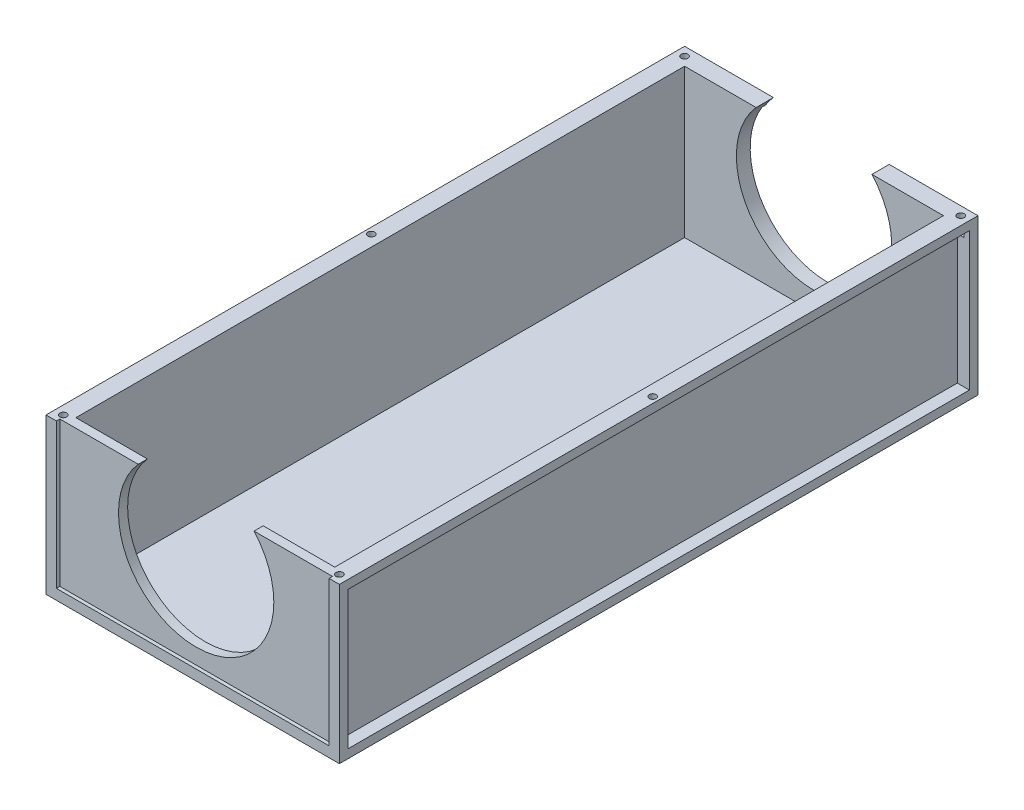
from build123d import *

# Parameters (mm, degrees)
SKETCH_1_R           = 50
SKETCH_1_R_2         = 42.55
EXTRUDE_1_DEPTH      = 50
SKETCH_3_R           = 45
SKETCH_3_R_2         = 37.55
EXTRUDE_2_DEPTH      = 50
EXTRUDE_START        = -50
EXTRUDE_3_DEPTH      = 50
SKETCH_8_R           = 37.55
EXTRUDE_4_DEPTH      = 50
SKETCH_4_W           = 700
SKETCH_4_H           = 3700
EXTRUDE_5_DEPTH      = 300
SKETCH_12_W          = 500
SKETCH_12_H          = 1000
EXTRUDE_6_DEPTH      = 300
SKETCH_16_W          = 500
SKETCH_16_H          = 2700
EXTRUDE_8_DEPTH      = 300
SKETCH_17_W          = 100
SKETCH_17_H          = 100
EXTRUDE_9_DEPTH      = 600
SKETCH_18_W          = 100
SKETCH_18_H          = 100
EXTRUDE_10_DEPTH     = 600
SKETCH_19_W          = 100
SKETCH_19_H          = 100
EXTRUDE_11_DEPTH     = 3500
SKETCH_20_R          = 25
CUT_EXTRUDE_5_DEPTH  = 20
SKETCH_21_R          = 52.5
SKETCH_21_R_2        = 42.55
EXTRUDE_12_DEPTH     = 50
CUT_EXTRUDE_START    = -356
CUT_EXTRUDE_6_DEPTH  = 356
SKETCH_23_W          = 47.45
SKETCH_23_H          = 50
EXTRUDE_13_DEPTH     = 20
CUT_EXTRUDE_8_DEPTH  = 611
SKETCH_26_W          = 52.45
SKETCH_26_H          = 50
EXTRUDE_14_DEPTH     = 20
SKETCH_27_R          = 6
CUT_EXTRUDE_9_DEPTH  = 20
SKETCH_28_R          = 6
CUT_EXTRUDE_10_DEPTH = 20
EXTRUDE_START_2      = -53
EXTRUDE_15_DEPTH     = 53
EXTRUDE_START_3      = 3
EXTRUDE_16_DEPTH     = 3
EXTRUDE_17_DEPTH     = 3
EXTRUDE_18_DEPTH     = 53
SKETCH_31_W          = 3500
SKETCH_31_H          = 500
EXTRUDE_19_DEPTH     = 100
SKETCH_33_W          = 500
SKETCH_33_H          = 3700
EXTRUDE_20_DEPTH     = 300
EXTRUDE_21_DEPTH     = 100
SKETCH_35_W          = 1500
SKETCH_35_H          = 600
EXTRUDE_22_DEPTH     = 100
SKETCH_36_W          = 1500
SKETCH_36_H          = 600
EXTRUDE_23_DEPTH     = 100
SKETCH_37_W          = 3600
SKETCH_37_H          = 800
CUT_EXTRUDE_11_DEPTH = 70
SKETCH_38_W          = 1580
SKETCH_38_H          = 780
CUT_EXTRUDE_15_DEPTH = 20
SKETCH_39_W          = 3600
SKETCH_39_H          = 800
CUT_EXTRUDE_16_DEPTH = 70
SKETCH_40_W          = 1580
SKETCH_40_H          = 780
CUT_EXTRUDE_17_DEPTH = 20
SKETCH_43_R          = 20
CUT_EXTRUDE_20_DEPTH = 100
CUT_EXTRUDE_22_DEPTH = 260
SKETCH_44_W          = 1500
SKETCH_44_H          = 3527
CUT_EXTRUDE_24_DEPTH = 983
CUT_EXTRUDE_25_DEPTH = 260
SKETCH_49_W          = 1580
SKETCH_49_H          = 840
CUT_EXTRUDE_26_DEPTH = 20
SKETCH_52_R          = 450
CUT_EXTRUDE_30_DEPTH = 492
SKETCH_53_R          = 450
CUT_EXTRUDE_31_DEPTH = 492


with BuildPart() as part:
    # 草图1 → 凸台-拉伸1 (new body)
    with BuildSketch(Plane.XY):
        Circle(SKETCH_1_R)
        Circle(SKETCH_1_R_2, mode=Mode.SUBTRACT)
    extrude(amount=EXTRUDE_1_DEPTH)

    # 草图7 → 凸台-拉伸3 (add)
    with BuildSketch(Plane.XY.offset(50).offset(EXTRUDE_START)):
        with BuildLine():
            ThreePointArc((50, 0), (0, -50), (-50, 0))
            Line((-50, 0), (-250, -900))
            Line((-250, -900), (250, -900))
            Line((250, -900), (50, 0))
        make_face()
    extrude(amount=EXTRUDE_3_DEPTH)



with BuildPart() as body_2:
    # 草图3 → 凸台-拉伸2 (new body)
    with BuildSketch(Plane(origin=(0, 0, -3374), x_dir=(-1, 0, 0), z_dir=(0, 0, -1))):
        Circle(SKETCH_3_R)
        Circle(SKETCH_3_R_2, mode=Mode.SUBTRACT)
    extrude(amount=EXTRUDE_2_DEPTH)

    # 草图8 → 凸台-拉伸4 (add)
    with BuildSketch(Plane(origin=(0, 0, -3424), x_dir=(-1, 0, 0), z_dir=(0, 0, -1))):
        with BuildLine():
            Line((-43.888190419, 9.941164005), (-250, -900))
            Line((-250, -900), (250, -900))
            Line((250, -900), (43.888190419, 9.941164005))
            ThreePointArc((43.888190419, 9.941164005), (0, 45), (-43.888190419, 9.941164005))
        make_face()
        Circle(SKETCH_8_R, mode=Mode.SUBTRACT)
    extrude(amount=-EXTRUDE_4_DEPTH)


with BuildPart() as part_1:
    add(part.part)

    add(body_2.part)  # 凸台-拉伸5 merges body 2
    # 草图4 → 凸台-拉伸5 (add)
    with BuildSketch(Plane(origin=(0, -900, 0), x_dir=(1, 0, 0), z_dir=(0, 1, 0))):
        with Locations((0, 1724)):
            Rectangle(SKETCH_4_W, SKETCH_4_H)
    extrude(amount=-EXTRUDE_5_DEPTH)

    # 草图12 → 凸台-拉伸6 (add)
    with BuildSketch(Plane(origin=(0, -900, 0), x_dir=(1, 0, 0), z_dir=(0, 1, 0))):
        with Locations((600, 374)):
            Rectangle(SKETCH_12_W, SKETCH_12_H)
    extrude(amount=-EXTRUDE_6_DEPTH)

    # 草图16 → 凸台-拉伸8 (add)
    with BuildSketch(Plane(origin=(0, -900, 0), x_dir=(1, 0, 0), z_dir=(0, 1, 0))):
        with Locations((600, 2224)):
            Rectangle(SKETCH_16_W, SKETCH_16_H)
    extrude(amount=-EXTRUDE_8_DEPTH)

    # 草图17 → 凸台-拉伸9 (add)
    with BuildSketch(Plane(origin=(0, -900, 0), x_dir=(1, 0, 0), z_dir=(0, 1, 0))):
        with Locations((800, 3524)):
            Rectangle(SKETCH_17_W, SKETCH_17_H)
    extrude(amount=EXTRUDE_9_DEPTH)

    # 草图18 → 凸台-拉伸10 (add)
    with BuildSketch(Plane(origin=(0, -900, 0), x_dir=(1, 0, 0), z_dir=(0, 1, 0))):
        with Locations((800, -76)):
            Rectangle(SKETCH_18_W, SKETCH_18_H)
    extrude(amount=EXTRUDE_10_DEPTH)

    # 草图19 → 凸台-拉伸11 (add)
    with BuildSketch(Plane.XY.offset(-3474)):
        with Locations((800, -350)):
            Rectangle(SKETCH_19_W, SKETCH_19_H)
    extrude(amount=EXTRUDE_11_DEPTH)

    # 草图20 → 切除-拉伸5 (cut)
    with BuildSketch(Plane.ZY.offset(-750)):
        with Locations((-3424, -350)):
            Circle(SKETCH_20_R)
    extrude(amount=-CUT_EXTRUDE_5_DEPTH, mode=Mode.SUBTRACT)

    # 草图21 → 凸台-拉伸12 (add)
    with BuildSketch(Plane.XY.offset(50).offset(EXTRUDE_START)):
        Circle(SKETCH_21_R)
        Circle(SKETCH_21_R_2, mode=Mode.SUBTRACT)
    extrude(amount=EXTRUDE_12_DEPTH)

    # 草图22 → 切除-拉伸6 (cut)
    with BuildSketch(Plane.XY.offset(50).offset(CUT_EXTRUDE_START)):
        with BuildLine():
            Line((-52.5, 0), (52.5, 0))
            ThreePointArc((52.5, 0), (0, 52.5), (-52.5, 0))
        make_face()
    extrude(amount=CUT_EXTRUDE_6_DEPTH, mode=Mode.SUBTRACT)

    # 草图23 → 凸台-拉伸13 (add)
    with BuildSketch(Plane(origin=(0, 0, 0), x_dir=(1, 0, 0), z_dir=(0, 1, 0))):
        with Locations((-66.275, -25)):
            Rectangle(SKETCH_23_W, SKETCH_23_H)
        with Locations((66.275, -25)):
            Rectangle(SKETCH_23_W, SKETCH_23_H)
    extrude(amount=-EXTRUDE_13_DEPTH)

    # 草图24 → 切除-拉伸8 (cut)
    with BuildSketch(Plane(origin=(0, 0, -3424), x_dir=(-1, 0, 0), z_dir=(0, 0, -1))):
        with BuildLine():
            Line((-55, 0), (55, 0))
            ThreePointArc((55, 0), (0, 55), (-55, 0))
        make_face()
    extrude(amount=-CUT_EXTRUDE_8_DEPTH, mode=Mode.SUBTRACT)

    # 草图26 → 凸台-拉伸14 (add)
    with BuildSketch(Plane(origin=(0, 0, 0), x_dir=(1, 0, 0), z_dir=(0, 1, 0))):
        with Locations((-63.775, 3399)):
            Rectangle(SKETCH_26_W, SKETCH_26_H)
        with Locations((63.775, 3399)):
            Rectangle(SKETCH_26_W, SKETCH_26_H)
    extrude(amount=-EXTRUDE_14_DEPTH)

    # 草图27 → 切除-拉伸9 (cut)
    with BuildSketch(Plane(origin=(0, 0, 0), x_dir=(1, 0, 0), z_dir=(0, 1, 0))):
        with Locations(Location((-75, -12.5, 0), (0, 0, 270))):
            Circle(SKETCH_27_R)
        with Locations(Location((-75, -37.5, 0), (0, 0, 270))):
            Circle(SKETCH_27_R)
        with Locations(Location((75, -37.5, 0), (0, 0, 90))):
            Circle(SKETCH_27_R)
        with Locations(Location((75, -12.5, 0), (0, 0, 90))):
            Circle(SKETCH_27_R)
    extrude(amount=-CUT_EXTRUDE_9_DEPTH, mode=Mode.SUBTRACT)

    # 草图28 → 切除-拉伸10 (cut)
    with BuildSketch(Plane(origin=(0, 0, 0), x_dir=(1, 0, 0), z_dir=(0, 1, 0))):
        with Locations(Location((-75, 3411.5, 0), (0, 0, 270))):
            Circle(SKETCH_28_R)
        with Locations(Location((-75, 3386.5, 0), (0, 0, 270))):
            Circle(SKETCH_28_R)
        with Locations(Location((75, 3386.5, 0), (0, 0, 90))):
            Circle(SKETCH_28_R)
        with Locations(Location((75, 3411.5, 0), (0, 0, 90))):
            Circle(SKETCH_28_R)
    extrude(amount=-CUT_EXTRUDE_10_DEPTH, mode=Mode.SUBTRACT)

    # 草图29 → 凸台-拉伸15 (add)
    with BuildSketch(Plane.XY.offset(50).offset(EXTRUDE_START_2)):
        with BuildLine():
            Line((-52.5, 0), (-42.55, 0))
            ThreePointArc((-42.55, 0), (0, -42.55), (42.55, 0))
            Line((42.55, 0), (52.5, 0))
            ThreePointArc((52.5, 0), (0, -52.5), (-52.5, 0))
        make_face()
    extrude(amount=EXTRUDE_15_DEPTH)

    # 草图30 → 凸台-拉伸16 (add)
    with BuildSketch(Plane.XY.offset(-3374).offset(EXTRUDE_START_3)):
        with BuildLine():
            Line((-45, 0), (-37.55, 0))
            ThreePointArc((-37.55, 0), (0, -37.55), (37.55, 0))
            Line((37.55, 0), (45, 0))
            ThreePointArc((45, 0), (0, -45), (-45, 0))
        make_face()
    extrude(amount=-EXTRUDE_16_DEPTH)

    # 草图29<2> → 凸台-拉伸17 (add)
    with BuildSketch(Plane.XY.offset(50)):
        with BuildLine():
            Line((-52.5, 0), (-42.55, 0))
            ThreePointArc((-42.55, 0), (0, -42.55), (42.55, 0))
            Line((42.55, 0), (52.5, 0))
            ThreePointArc((52.5, 0), (0, -52.5), (-52.5, 0))
        make_face()
    extrude(amount=EXTRUDE_17_DEPTH)

    # 草图30<2> → 凸台-拉伸18 (add)
    with BuildSketch(Plane.XY.offset(-3374)):
        with BuildLine():
            Line((-45, 0), (-37.55, 0))
            ThreePointArc((-37.55, 0), (0, -37.55), (37.55, 0))
            Line((37.55, 0), (45, 0))
            ThreePointArc((45, 0), (0, -45), (-45, 0))
        make_face()
    extrude(amount=-EXTRUDE_18_DEPTH)

    # 草图31 → 凸台-拉伸19 (add)
    with BuildSketch(Plane.ZY.offset(-750)):
        with Locations((-1724, -650)):
            Rectangle(SKETCH_31_W, SKETCH_31_H)
    extrude(amount=-EXTRUDE_19_DEPTH)

    # 草图33 → 凸台-拉伸20 (add)
    with BuildSketch(Plane(origin=(0, -900, 0), x_dir=(1, 0, 0), z_dir=(0, 1, 0))):
        with Locations((-600, 1724)):
            Rectangle(SKETCH_33_W, SKETCH_33_H)
    extrude(amount=-EXTRUDE_20_DEPTH)

    # 草图34 → 凸台-拉伸21 (add)
    with BuildSketch(Plane.ZY.offset(850)):
        Polygon((126, -300), (126, -900), (126, -1200), (-3574, -1200), (-3574, -900), (-3574, -300), align=None)
    extrude(amount=-EXTRUDE_21_DEPTH)

    # 草图35 → 凸台-拉伸22 (add)
    with BuildSketch(Plane(origin=(0, 0, -3574), x_dir=(-1, 0, 0), z_dir=(0, 0, -1))):
        with Locations((0, -600)):
            Rectangle(SKETCH_35_W, SKETCH_35_H)
    extrude(amount=-EXTRUDE_22_DEPTH)

    # 草图36 → 凸台-拉伸23 (add)
    with BuildSketch(Plane.XY.offset(126)):
        with Locations((0, -600)):
            Rectangle(SKETCH_36_W, SKETCH_36_H)
    extrude(amount=-EXTRUDE_23_DEPTH)

    # 草图37 → 切除-拉伸11 (cut)
    with BuildSketch(Plane.ZY.offset(850)):
        with Locations((-1724, -750)):
            Rectangle(SKETCH_37_W, SKETCH_37_H)
    extrude(amount=-CUT_EXTRUDE_11_DEPTH, mode=Mode.SUBTRACT)

    # 草图38 → 切除-拉伸15 (cut)
    with BuildSketch(Plane(origin=(0, 0, -3574), x_dir=(-1, 0, 0), z_dir=(0, 0, -1))):
        with Locations((0, -750)):
            Rectangle(SKETCH_38_W, SKETCH_38_H)
    extrude(amount=-CUT_EXTRUDE_15_DEPTH, mode=Mode.SUBTRACT)

    # 草图39 → 切除-拉伸16 (cut)
    with BuildSketch(Plane(origin=(850, 0, 0), x_dir=(0, 0, -1), z_dir=(1, 0, 0))):
        with Locations((1724, -750)):
            Rectangle(SKETCH_39_W, SKETCH_39_H)
    extrude(amount=-CUT_EXTRUDE_16_DEPTH, mode=Mode.SUBTRACT)

    # 草图40 → 切除-拉伸17 (cut)
    with BuildSketch(Plane.XY.offset(126)):
        with Locations((0, -750)):
            Rectangle(SKETCH_40_W, SKETCH_40_H)
    extrude(amount=-CUT_EXTRUDE_17_DEPTH, mode=Mode.SUBTRACT)

    # 草图43 → 切除-拉伸20 (cut)
    with BuildSketch(Plane(origin=(0, -300, 0), x_dir=(1, 0, 0), z_dir=(0, 1, 0))):
        with Locations(Location((800, 3524, 0), (0, 0, 270))):
            Circle(SKETCH_43_R)
        with Locations(Location((-800, 3524, 0), (0, 0, 270))):
            Circle(SKETCH_43_R)
        with Locations(Location((815, 1724, 0), (0, 0, 270))):
            Circle(SKETCH_43_R)
        with Locations(Location((-815, 1724, 0), (0, 0, 270))):
            Circle(SKETCH_43_R)
        with Locations(Location((800, -76, 0), (0, 0, 180))):
            Circle(SKETCH_43_R)
        with Locations((-800, -76)):
            Circle(SKETCH_43_R)
    extrude(amount=-CUT_EXTRUDE_20_DEPTH, mode=Mode.SUBTRACT)

    # 草图45 → 切除-拉伸22 (cut)
    with BuildSketch(Plane(origin=(0, -900, 0), x_dir=(1, 0, 0), z_dir=(0, 1, 0))):
        Polygon((-750, 3474), (-750, -26), (-250, -26), (-250, 0), (250, 0), (250, -26), (750, -26), (750, 3474), align=None)
    extrude(amount=-CUT_EXTRUDE_22_DEPTH, mode=Mode.SUBTRACT)


with BuildPart() as cut_extrude_22_piece_1:
    # of the separate pieces the step leaves, piece 1, a body of its own (cut_extrude_22_pieces)
    add(part_1.part.solids().sort_by_distance((850, -1200, 126))[0])


with BuildPart() as cut_extrude_22_piece_2:
    # of the separate pieces the step leaves, piece 2, a body of its own (cut_extrude_22_pieces)
    add(part_1.part.solids().sort_by_distance((-250, -900, -3424))[0])


with BuildPart() as cut_extrude_24_tool:
    # 草图44 → 切除-拉伸24 (new body)
    with BuildSketch(Plane(origin=(0, -900, 0), x_dir=(1, 0, 0), z_dir=(0, 1, 0))):
        with Locations((0, 1710.5)):
            Rectangle(SKETCH_44_W, SKETCH_44_H)
    extrude(amount=CUT_EXTRUDE_24_DEPTH)


with BuildPart() as cut_extrude_22_piece_1_1:
    add(cut_extrude_22_piece_1.part)

    # 切除-拉伸24: cut by cut_extrude_24_tool
    add(cut_extrude_24_tool.part, mode=Mode.SUBTRACT)

    # 草图48 → 切除-拉伸25 (cut)
    with BuildSketch(Plane(origin=(0, -900, 0), x_dir=(1, 0, 0), z_dir=(0, 1, 0))):
        Polygon((250, -26), (250, 0), (-250, 0), (-250, -26), (-750, -26), (-750, -53), (750, -53), (750, -26), align=None)
    extrude(amount=-CUT_EXTRUDE_25_DEPTH, mode=Mode.SUBTRACT)

    # 草图49 → 切除-拉伸26 (cut)
    with BuildSketch(Plane.XY.offset(126)):
        with Locations((0, -720)):
            Rectangle(SKETCH_49_W, SKETCH_49_H)
    extrude(amount=-CUT_EXTRUDE_26_DEPTH, mode=Mode.SUBTRACT)

    # 草图52 → 切除-拉伸30 (cut)
    with BuildSketch(Plane.XY.offset(-3574)):
        with Locations((0, -600)):
            Circle(SKETCH_52_R)
    extrude(amount=CUT_EXTRUDE_30_DEPTH, mode=Mode.SUBTRACT)

    # 草图53 → 切除-拉伸31 (cut)
    with BuildSketch(Plane.XY.offset(126)):
        with Locations((0, -600)):
            Circle(SKETCH_53_R)
    extrude(amount=-CUT_EXTRUDE_31_DEPTH, mode=Mode.SUBTRACT)


with BuildPart() as cut_extrude_22_piece_2_1:
    add(cut_extrude_22_piece_2.part)

    # 切除-拉伸24: cut by cut_extrude_24_tool
    add(cut_extrude_24_tool.part, mode=Mode.SUBTRACT)


solid = cut_extrude_22_piece_1_1.part
